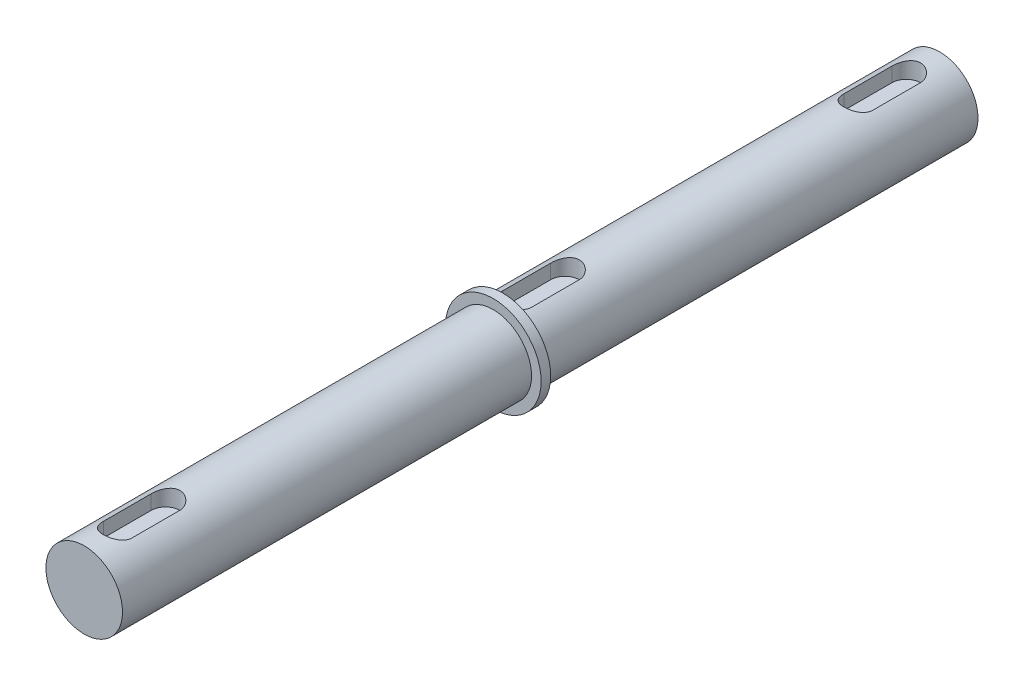
from build123d import *

# Parameters (mm, degrees)
SKETCH1_R           = 4
BOSS_EXTRUDE1_DEPTH = 45.65
SKETCH2_R           = 5
BOSS_EXTRUDE2_DEPTH = 1
SKETCH3_R           = 4
BOSS_EXTRUDE3_DEPTH = 42.74
CUT_EXTRUDE1_DEPTH  = 1.8


with BuildPart() as part:
    # Sketch1 → Boss-Extrude1 (new body)
    with BuildSketch(Plane.XY):
        Circle(SKETCH1_R)
    extrude(amount=BOSS_EXTRUDE1_DEPTH)

    # Sketch2 → Boss-Extrude2 (add)
    with BuildSketch(Plane.XY.offset(45.65)):
        Circle(SKETCH2_R)
    extrude(amount=BOSS_EXTRUDE2_DEPTH)

    # Sketch3 → Boss-Extrude3 (add)
    with BuildSketch(Plane.XY.offset(46.65)):
        Circle(SKETCH3_R)
    extrude(amount=BOSS_EXTRUDE3_DEPTH)

    # Sketch4 → Cut-Extrude1 (cut)
    with BuildSketch(Plane(origin=(0, 4, 0), x_dir=(1, 0, 0), z_dir=(0, 1, 0))):
        with BuildLine():
            Line((1.5, -3.5), (1.5, -8.5))
            ThreePointArc((1.5, -8.5), (0, -10), (-1.5, -8.5))
            Line((-1.5, -8.5), (-1.5, -3.5))
            ThreePointArc((-1.5, -3.5), (0, -2), (1.5, -3.5))
        make_face()
        with BuildLine():
            Line((1.5, -39.15), (1.5, -44.15))
            ThreePointArc((1.5, -44.15), (0, -45.65), (-1.5, -44.15))
            Line((-1.5, -44.15), (-1.5, -39.15))
            ThreePointArc((-1.5, -39.15), (0, -37.65), (1.5, -39.15))
        make_face()
        with BuildLine():
            Line((1.5, -80.89), (1.5, -85.89))
            ThreePointArc((1.5, -85.89), (0, -87.39), (-1.5, -85.89))
            Line((-1.5, -85.89), (-1.5, -80.89))
            ThreePointArc((-1.5, -80.89), (0, -79.39), (1.5, -80.89))
        make_face()
    extrude(amount=-CUT_EXTRUDE1_DEPTH, mode=Mode.SUBTRACT)


solid = part.part
